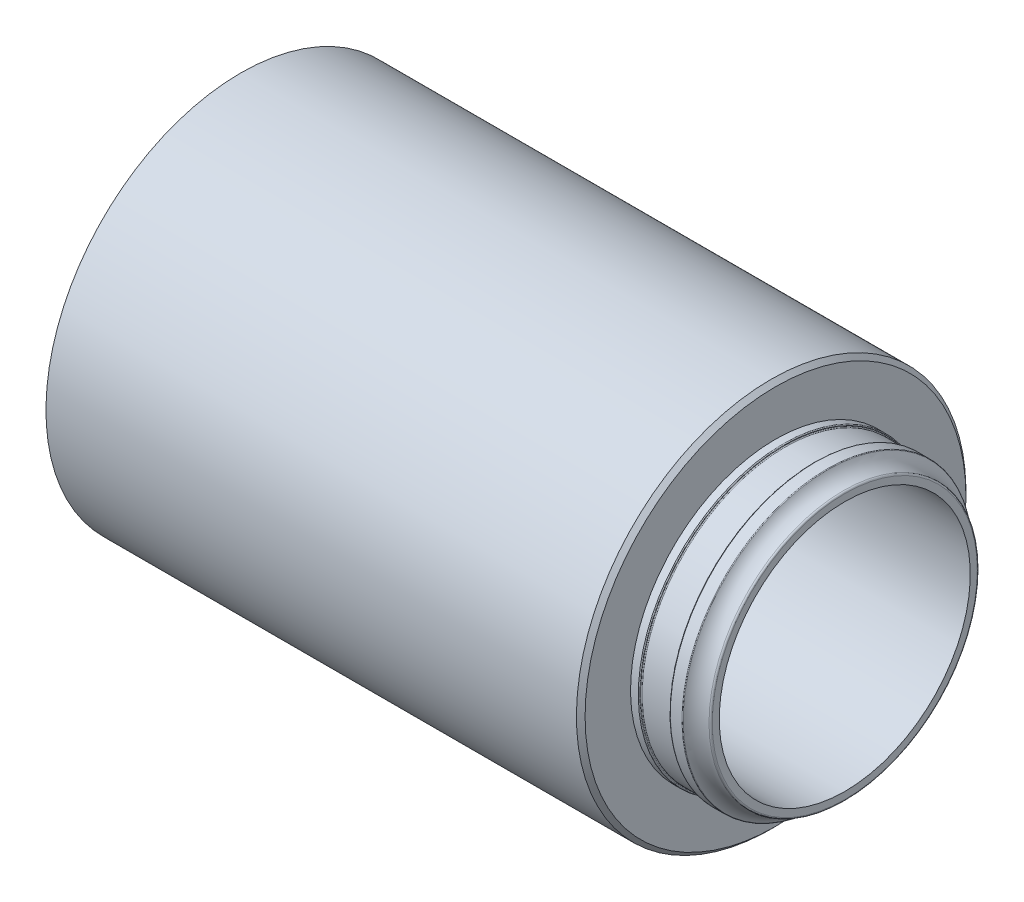
from build123d import *


with BuildPart() as part:
    # Sketch1 → Revolve1 (revolve)
    with BuildSketch(Plane.XY):
        with BuildLine():
            Line((437.264284999, 33.5), (434.584463757, 33.5))
            ThreePointArc((434.584463757, 33.5), (434.443042401, 33.441421356), (434.384463757, 33.3))
            Line((434.384463757, 33.3), (434.384463757, 33.2))
            ThreePointArc((434.384463757, 33.2), (434.325885113, 33.058578644), (434.184463757, 33))
            Line((434.184463757, 33), (427.584463757, 33))
            ThreePointArc((427.584463757, 33), (427.443042401, 33.058578644), (427.384463757, 33.2))
            Line((427.384463757, 33.2), (427.384463757, 33.3))
            ThreePointArc((427.384463757, 33.3), (427.325885113, 33.441421356), (427.184463757, 33.5))
            Line((427.184463757, 33.5), (425.384463757, 33.5))
            Line((425.384463757, 33.5), (425.384463757, 44))
            Line((425.384463757, 44), (424.384463757, 45))
            Line((424.384463757, 45), (411.824463757, 45))
            Line((411.824463757, 45), (391.824463757, 45))
            Line((391.824463757, 45), (301.824463757, 45))
            Line((301.824463757, 45), (301.824463757, 29))
            Line((301.824463757, 29), (441.384463757, 29))
            Line((441.384463757, 29), (441.384463757, 30.615822229))
            ThreePointArc((441.384463757, 30.615822229), (441.281521436, 30.883696706), (441.02568008, 31.013693081))
            ThreePointArc((441.02568008, 31.013693081), (438.939166095, 31.763093605), (437.439685601, 33.396096976))
            ThreePointArc((437.439685601, 33.396096976), (437.366217832, 33.472074686), (437.264284999, 33.5))
        make_face()
    revolve(axis=Axis((597.174463757, 0, 0), (-1, 0, 0)))


solid = part.part
